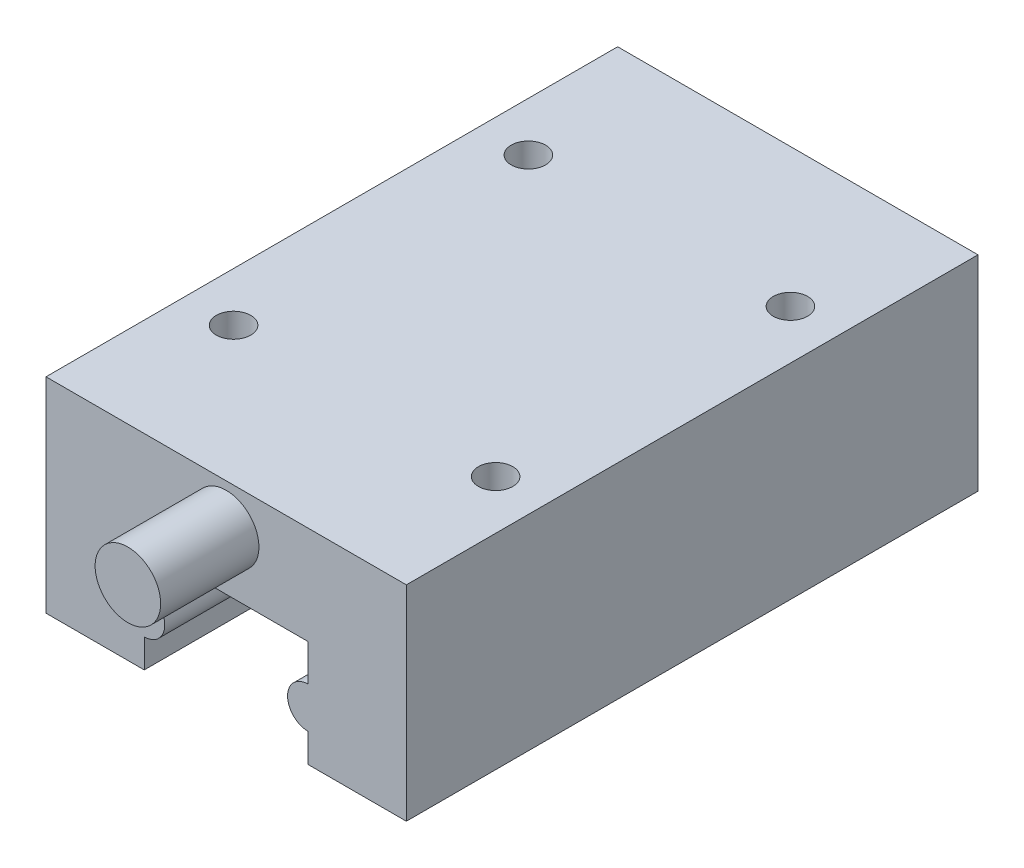
from build123d import *

# Parameters (mm, degrees)
EXTRUDE1_DEPTH        = 34.9
SKETCH2_R             = 4
EXTRUDE2_DEPTH        = 12
M5_TAPPED_HOLE1_D     = 4.2
M5_TAPPED_HOLE1_DEPTH = 12.4
M5_TAPPED_HOLE1_TIP   = 1.2618073


with BuildPart() as part:
    # Sketch1 → Extrude1 (new, symmetric)
    with BuildSketch(Plane.XY):
        with BuildLine():
            Line((32, -25), (44, -25))
            Line((44, -25), (44, 0))
            Line((44, 0), (0, 0))
            Line((0, 0), (0, -25))
            Line((0, -25), (12, -25))
            Line((12, -25), (12, -21.5))
            ThreePointArc((12, -21.5), (14.5, -19), (12, -16.5))
            Line((12, -16.5), (12, -12))
            Line((12, -12), (32, -12))
            Line((32, -12), (32, -16.5))
            ThreePointArc((32, -16.5), (29.5, -19), (32, -21.5))
            Line((32, -21.5), (32, -25))
        make_face()
    extrude(amount=EXTRUDE1_DEPTH, both=True)

    # Sketch2 → Extrude2 (add)
    with BuildSketch(Plane.XY.offset(34.9)):
        with Locations((22, -5)):
            Circle(SKETCH2_R)
    extrude(amount=EXTRUDE2_DEPTH)

    # M5 Tapped Hole1
    with Locations(Plane(origin=(6, 0, 18), x_dir=(0, 0, 1), z_dir=(0, 1, 0))):
        with Locations((0, 0), (0, 32), (-36, 0), (-36, 32)):
            Hole(M5_TAPPED_HOLE1_D / 2, depth=M5_TAPPED_HOLE1_DEPTH)
            with Locations((0, 0, -(M5_TAPPED_HOLE1_DEPTH + M5_TAPPED_HOLE1_TIP / 2))):  # 118° drill point
                Cone(0, M5_TAPPED_HOLE1_D / 2, M5_TAPPED_HOLE1_TIP, mode=Mode.SUBTRACT)


solid = part.part
